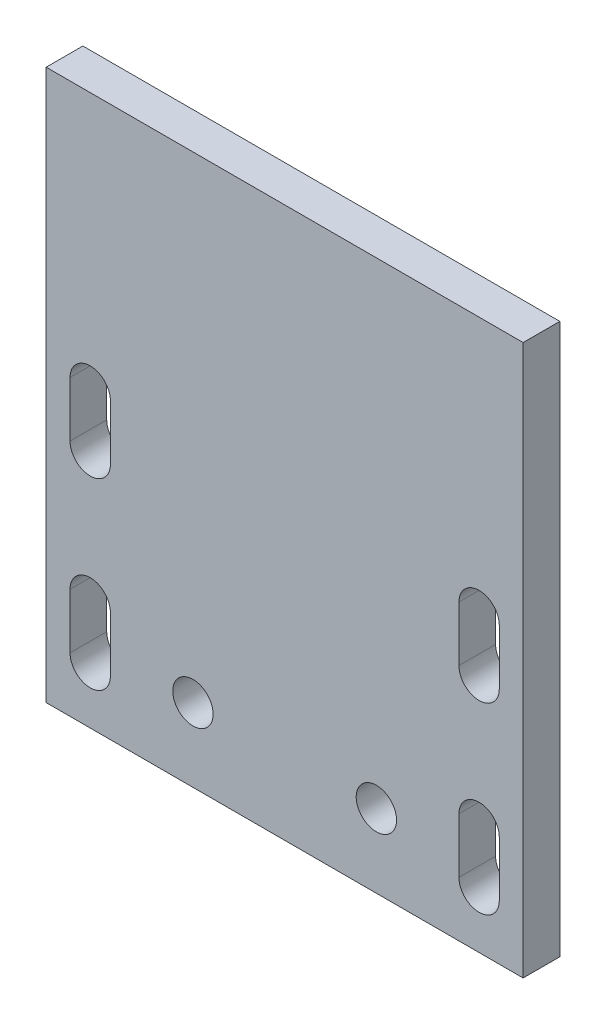
from build123d import *

# Parameters (mm, degrees)
SKETCH1_W                  = 130
SKETCH1_H                  = 130
BOSS_EXTRUDE1_DEPTH        = 10
F_11_0_11_DIAMETER_HOLE1_D = 11
SKETCH4_W                  = 130
SKETCH4_H                  = 10
BOSS_EXTRUDE2_DEPTH        = 20
M6_CLEARANCE_HOLE1_D       = 7
CUT_EXTRUDE1_DEPTH         = 199.746069144


with BuildPart() as part:
    # Sketch1 → Boss-Extrude1 (new body)
    with BuildSketch(Plane.XY):
        with Locations((65, 65)):
            Rectangle(SKETCH1_W, SKETCH1_H)
    extrude(amount=BOSS_EXTRUDE1_DEPTH)

    # Ø11.0 (11) Diameter Hole1 (through all)
    with Locations(Plane.XY.offset(10)):
        with Locations((40, 20), (90, 20)):
            Hole(F_11_0_11_DIAMETER_HOLE1_D / 2)

    # Sketch4 → Boss-Extrude2 (add)
    with BuildSketch(Plane(origin=(0, 130, 0), x_dir=(1, 0, 0), z_dir=(0, 1, 0))):
        with Locations((65, -5)):
            Rectangle(SKETCH4_W, SKETCH4_H)
    extrude(amount=BOSS_EXTRUDE2_DEPTH)

    # M6 Clearance Hole1 (through all)
    with Locations(Plane(origin=(0, 0, 0), x_dir=(-1, 0, 0), z_dir=(0, 0, -1))):
        with Locations((-118, 68.5), (-118, 18.5), (-12, 68.5), (-12, 18.5)):
            Hole(M6_CLEARANCE_HOLE1_D / 2)

    # Sketch8 → Cut-Extrude1 (cut, through all)
    with BuildSketch(Plane(origin=(0, 0, 0), x_dir=(-1, 0, 0), z_dir=(0, 0, -1))):
        with BuildLine():
            Line((-123.5, 15), (-123.5, 30))
            ThreePointArc((-123.5, 30), (-118, 35.5), (-112.5, 30))
            Line((-112.5, 30), (-112.5, 15))
            ThreePointArc((-112.5, 15), (-118, 9.5), (-123.5, 15))
        make_face()
        with BuildLine():
            Line((-123.5, 65), (-123.5, 80))
            ThreePointArc((-123.5, 80), (-118, 85.5), (-112.5, 80))
            Line((-112.5, 80), (-112.5, 65))
            ThreePointArc((-112.5, 65), (-118, 59.5), (-123.5, 65))
        make_face()
        with BuildLine():
            Line((-17.5, 65), (-17.5, 80))
            ThreePointArc((-17.5, 80), (-12, 85.5), (-6.5, 80))
            Line((-6.5, 80), (-6.5, 65))
            ThreePointArc((-6.5, 65), (-12, 59.5), (-17.5, 65))
        make_face()
        with BuildLine():
            Line((-17.5, 15), (-17.5, 30))
            ThreePointArc((-17.5, 30), (-12, 35.5), (-6.5, 30))
            Line((-6.5, 30), (-6.5, 15))
            ThreePointArc((-6.5, 15), (-12, 9.5), (-17.5, 15))
        make_face()
    extrude(amount=-CUT_EXTRUDE1_DEPTH, mode=Mode.SUBTRACT)


solid = part.part
